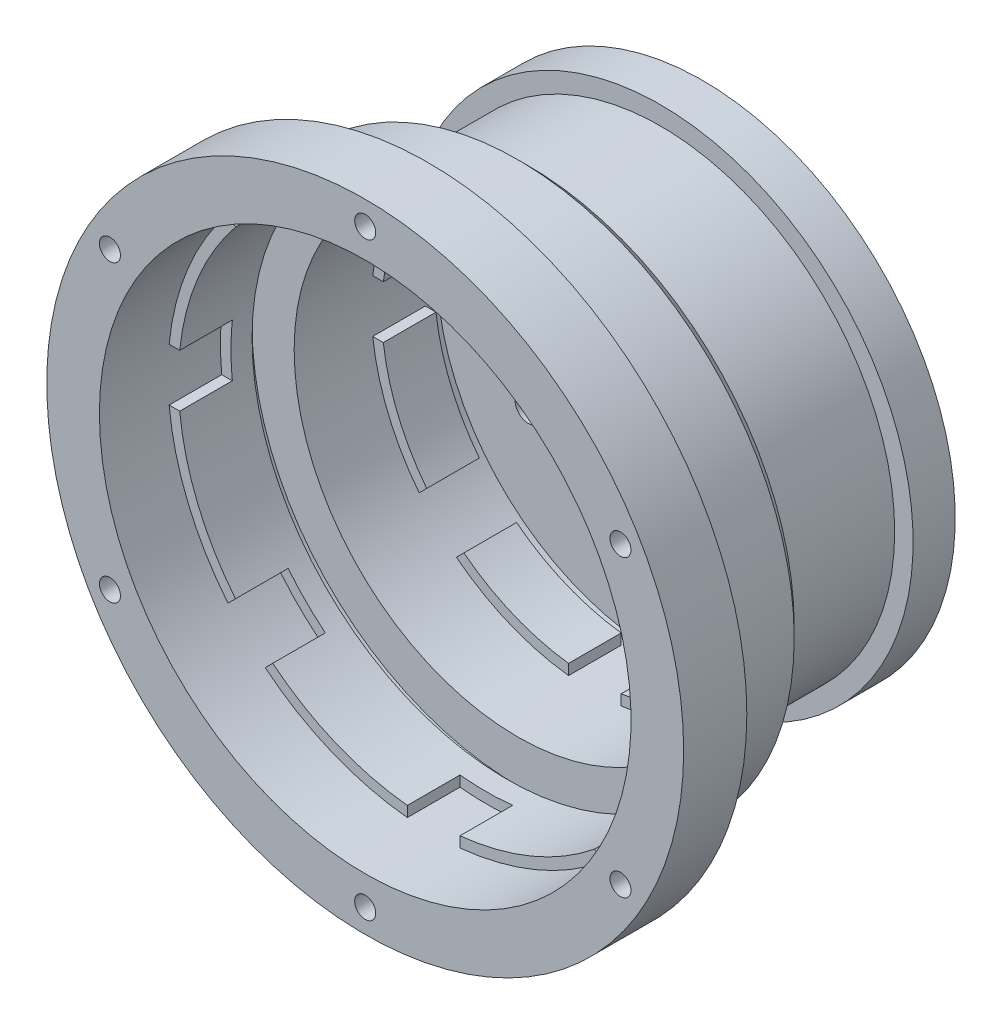
from build123d import *

# Parameters (mm, degrees)
CUT_EXTRUDE2_START  = -10
SKETCH3_R           = 40.5
CUT_EXTRUDE2_DEPTH  = 10
CUT_EXTRUDE3_START  = -10
CUT_EXTRUDE3_DEPTH  = 10
CIRPATTERN5_COUNT   = 8
CHAMFER1_SIZE       = 2
SKETCH4_R           = 48
SKETCH4_R_2         = 15
SKETCH4_R_3         = 2.5
BOSS_EXTRUDE1_DEPTH = 8
SKETCH7_R           = 60.5
SKETCH7_R_2         = 52.5
SKETCH7_R_3         = 2
BOSS_EXTRUDE2_DEPTH = 12


with BuildPart() as part:
    # Sketch1 → Revolve1 (revolve)
    with BuildSketch(Plane(origin=(0, 0, 0), x_dir=(1, 0, 0), z_dir=(0, 1, 0)), mode=Mode.PRIVATE) as revolve1_sk:
        Polygon((50.5, 3.905657953), (50.5, 16.905657953), (48.5, 16.905657953), (48.5, 30.905657953), (50.5, 30.905657953), (50.5, 32.905657953), (42.5, 32.905657953), (42.5, 47.535252784), (40.5, 47.535252784), (40.5, 57.535252784), (42.5, 57.535252784), (42.5, 60), (44.5, 60), (44.5, 34.905657953), (52.5, 34.905657953), (52.5, 3.905657953), align=None)
    revolve(revolve1_sk.sketch.rotate(Axis((0, 0, -60), (0, 0, 1)), 180), axis=Axis((0, 0, -60), (0, 0, 1)))

    # Sketch3 → Cut-Extrude2 (cut)
    with BuildSketch(Plane.XY.offset(-47.535252784).offset(CUT_EXTRUDE2_START)):
        with BuildLine():
            ThreePointArc((5, 42.20485754), (0, 42.5), (-5, 42.20485754))
            Line((-5, 42.20485754), (-5, 40.190172928))
            ThreePointArc((-5, 40.190172928), (0, 40.5), (5, 40.190172928))
            Line((5, 40.190172928), (5, 42.20485754))
        make_face()
        with BuildLine():
            ThreePointArc((33.378874872, 26.30780706), (30.0520382, 30.0520382), (26.30780706, 33.378874872))
            Line((26.30780706, 33.378874872), (24.883209909, 31.954277721))
            ThreePointArc((24.883209909, 31.954277721), (28.637824638, 28.637824638), (31.954277721, 24.883209909))
            Line((31.954277721, 24.883209909), (33.378874872, 26.30780706))
        make_face()
        with BuildLine():
            ThreePointArc((42.5, 0), (42.426150223, 2.504351666), (42.20485754, 5))
            Line((42.20485754, 5), (40.190172928, 5))
            ThreePointArc((40.190172928, 5), (40.422469022, 2.504795042), (40.5, 0))
            ThreePointArc((40.5, 0), (40.422469022, -2.504795042), (40.190172928, -5))
            Line((40.190172928, -5), (42.20485754, -5))
            ThreePointArc((42.20485754, -5), (42.426150223, -2.504351666), (42.5, 0))
        make_face()
        with BuildLine():
            ThreePointArc((26.30780706, -33.378874872), (30.0520382, -30.0520382), (33.378874872, -26.30780706))
            Line((33.378874872, -26.30780706), (31.954277721, -24.883209909))
            ThreePointArc((31.954277721, -24.883209909), (28.637824638, -28.637824638), (24.883209909, -31.954277721))
            Line((24.883209909, -31.954277721), (26.30780706, -33.378874872))
        make_face()
        with BuildLine():
            Line((-5, -40.190172928), (-5, -42.20485754))
            ThreePointArc((-5, -42.20485754), (0, -42.5), (5, -42.20485754))
            Line((5, -42.20485754), (5, -40.190172928))
            ThreePointArc((5, -40.190172928), (0, -40.5), (-5, -40.190172928))
        make_face()
        with BuildLine():
            Line((-31.954277721, -24.883209909), (-33.378874872, -26.30780706))
            ThreePointArc((-33.378874872, -26.30780706), (-30.0520382, -30.0520382), (-26.30780706, -33.378874872))
            Line((-26.30780706, -33.378874872), (-24.883209909, -31.954277721))
            ThreePointArc((-24.883209909, -31.954277721), (-28.637824638, -28.637824638), (-31.954277721, -24.883209909))
        make_face()
        with BuildLine():
            Line((-40.190172928, 5), (-42.20485754, 5))
            ThreePointArc((-42.20485754, 5), (-42.5, 0), (-42.20485754, -5))
            Line((-42.20485754, -5), (-40.190172928, -5))
            ThreePointArc((-40.190172928, -5), (-40.5, 0), (-40.190172928, 5))
        make_face()
        with BuildLine():
            Line((-24.883209909, 31.954277721), (-26.30780706, 33.378874872))
            ThreePointArc((-26.30780706, 33.378874872), (-30.0520382, 30.0520382), (-33.378874872, 26.30780706))
            Line((-33.378874872, 26.30780706), (-31.954277721, 24.883209909))
            ThreePointArc((-31.954277721, 24.883209909), (-28.637824638, 28.637824638), (-24.883209909, 31.954277721))
        make_face()
        Circle(SKETCH3_R)
    extrude(amount=CUT_EXTRUDE2_DEPTH, mode=Mode.SUBTRACT)

    # Sketch2 → Cut-Extrude3 (cut)
    with BuildSketch(Plane.XY.offset(-16.905657953).offset(CUT_EXTRUDE3_START)):
        with BuildLine():
            ThreePointArc((5, 50.251865637), (0, 50.5), (-5, 50.251865637))
            Line((-5, 50.251865637), (-5, 48.241579576))
            ThreePointArc((-5, 48.241579576), (0, 48.5), (5, 48.241579576))
            Line((5, 48.241579576), (5, 50.251865637))
        make_face()
    cut_extrude3 = extrude(amount=CUT_EXTRUDE3_DEPTH, mode=Mode.SUBTRACT)

    # CirPattern5: Cut-Extrude3 ×8 about axis
    cirpattern5_axis = Axis((0, 0, 0), (0, 0, 1))
    for i in range(1, CIRPATTERN5_COUNT):
        add(cut_extrude3.rotate(cirpattern5_axis, i * 360 / CIRPATTERN5_COUNT), mode=Mode.SUBTRACT)

    # Chamfer1
    chamfer1_edges = [part.edges().sort_by_distance(p)[0] for p in [
        (52.5, 0, -34.905657953),
    ]]
    chamfer(chamfer1_edges, length=CHAMFER1_SIZE)

    # Sketch4 → Boss-Extrude1 (add)
    with BuildSketch(Plane(origin=(0, 0, -60), x_dir=(-1, 0, 0), z_dir=(0, 0, -1))):
        Circle(SKETCH4_R)
        Circle(SKETCH4_R_2, mode=Mode.SUBTRACT)
        with Locations((0, 29)):
            Circle(SKETCH4_R_3, mode=Mode.SUBTRACT)
        with Locations((25.11473671, 14.5)):
            Circle(SKETCH4_R_3, mode=Mode.SUBTRACT)
        with Locations((25.11473671, -14.5)):
            Circle(SKETCH4_R_3, mode=Mode.SUBTRACT)
        with Locations((0, -29)):
            Circle(SKETCH4_R_3, mode=Mode.SUBTRACT)
        with Locations((-25.11473671, -14.5)):
            Circle(SKETCH4_R_3, mode=Mode.SUBTRACT)
        with Locations((-25.11473671, 14.5)):
            Circle(SKETCH4_R_3, mode=Mode.SUBTRACT)
    extrude(amount=BOSS_EXTRUDE1_DEPTH)

    # Sketch7 → Boss-Extrude2 (add)
    with BuildSketch(Plane.XY.offset(-3.905657953)):
        Circle(SKETCH7_R)
        Circle(SKETCH7_R_2, mode=Mode.SUBTRACT)
        with Locations((0, 56)):
            Circle(SKETCH7_R_3, mode=Mode.SUBTRACT)
        with Locations((48.497422612, 28)):
            Circle(SKETCH7_R_3, mode=Mode.SUBTRACT)
        with Locations((48.497422612, -28)):
            Circle(SKETCH7_R_3, mode=Mode.SUBTRACT)
        with Locations((0, -56)):
            Circle(SKETCH7_R_3, mode=Mode.SUBTRACT)
        with Locations((-48.497422612, -28)):
            Circle(SKETCH7_R_3, mode=Mode.SUBTRACT)
        with Locations((-48.497422612, 28)):
            Circle(SKETCH7_R_3, mode=Mode.SUBTRACT)
    extrude(amount=-BOSS_EXTRUDE2_DEPTH)


solid = part.part
